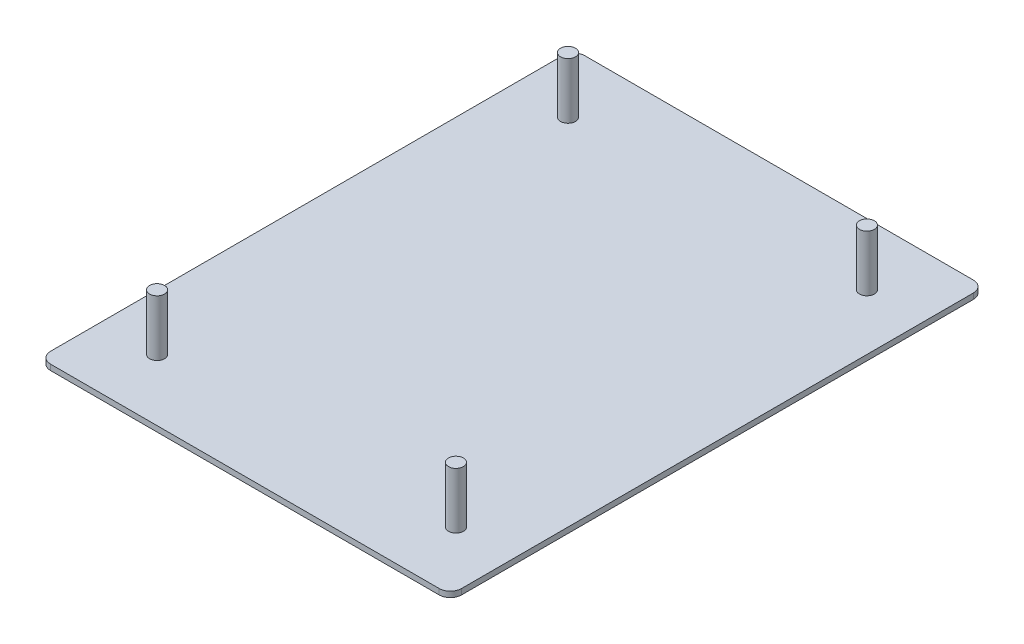
from build123d import *

# Parameters (mm, degrees)
SKETCH_1_W      = 110
SKETCH_1_H      = 143
EXTRUDE_1_DEPTH = 1.5
FILLET_1_R      = 3
SKETCH_2_R      = 2
EXTRUDE_2_DEPTH = 15


with BuildPart() as part:
    # 草图1 → 凸台-拉伸1 (new body)
    with BuildSketch(Plane(origin=(0, 0, 0), x_dir=(1, 0, 0), z_dir=(0, 1, 0))):
        with Locations((55, 71.5)):
            Rectangle(SKETCH_1_W, SKETCH_1_H)
    extrude(amount=EXTRUDE_1_DEPTH)

    # 圆角1
    fillet_1_edges = [part.edges().sort_by_distance(p)[0] for p in [
        (0, 0.75, -143),
        (110, 0.75, -143),
        (110, 0.75, 0),
        (0, 0.75, 0),
    ]]
    fillet(fillet_1_edges, radius=FILLET_1_R)

    # 草图2 → 凸台-拉伸2 (add)
    with BuildSketch(Plane(origin=(0, 1.5, 0), x_dir=(1, 0, 0), z_dir=(0, 1, 0))):
        with Locations(Location((15, 126.5, 0), (0, 0, 90))):
            Circle(SKETCH_2_R)
        with Locations(Location((95, 16.5, 0), (0, 0, 90))):
            Circle(SKETCH_2_R)
        with Locations(Location((15, 16.5, 0), (0, 0, 90))):
            Circle(SKETCH_2_R)
        with Locations(Location((95, 126.5, 0), (0, 0, 90))):
            Circle(SKETCH_2_R)
    extrude(amount=EXTRUDE_2_DEPTH)


solid = part.part
